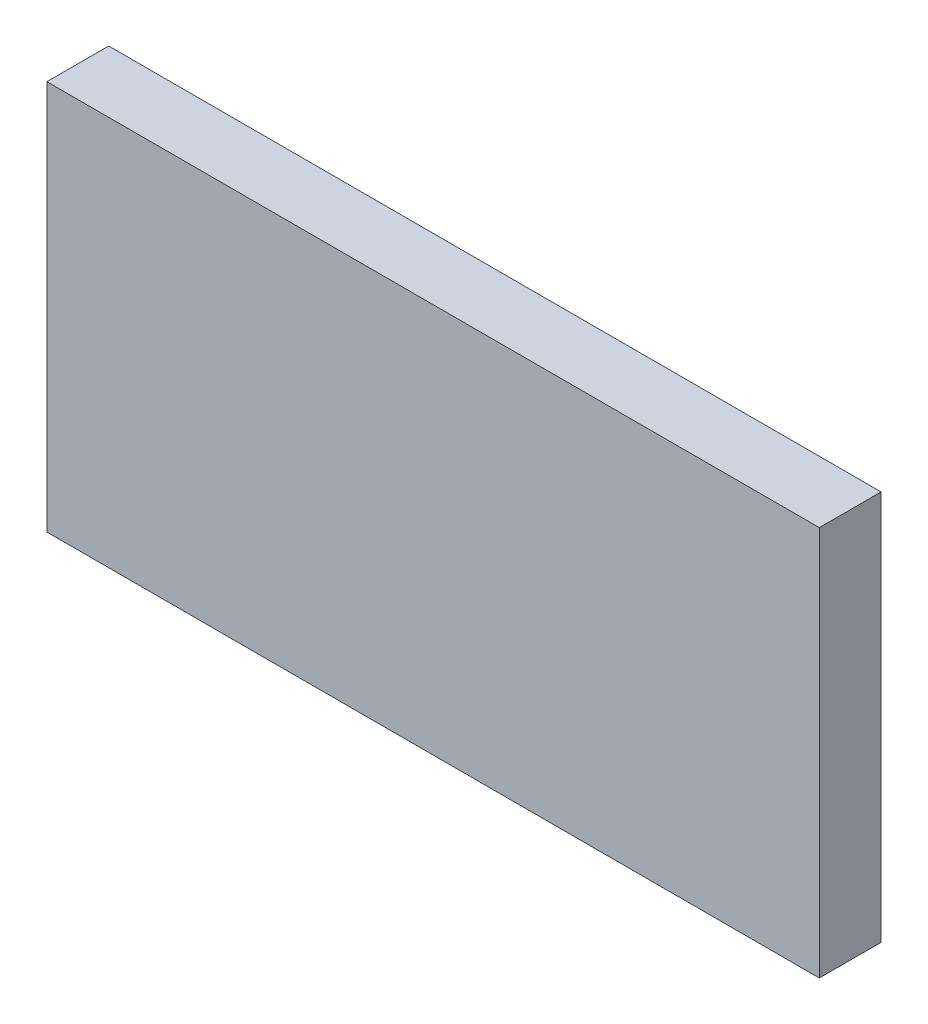
from build123d import *

# Parameters (mm, degrees)
SKETCH1_W           = 200
SKETCH1_H           = 101
BOSS_EXTRUDE1_DEPTH = 8


with BuildPart() as part:
    # Sketch1 → Boss-Extrude1 (new, symmetric)
    with BuildSketch(Plane.XY):
        Rectangle(SKETCH1_W, SKETCH1_H)
    extrude(amount=BOSS_EXTRUDE1_DEPTH, both=True)


solid = part.part
